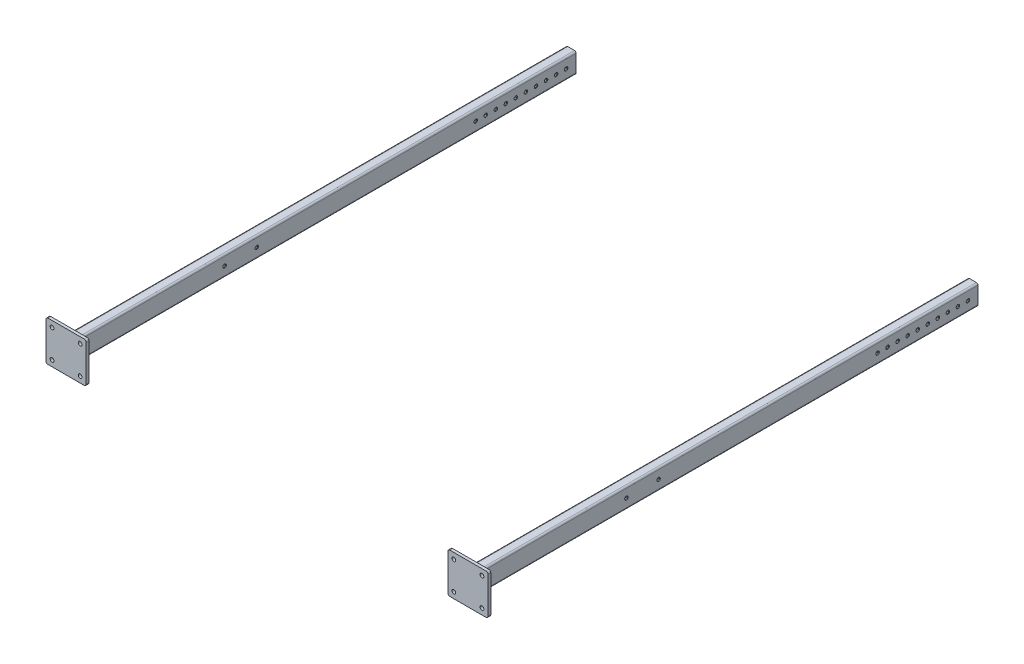
SolidWorks part; units mm, degrees
ref_plane "Front Plane" through (0, 0, 0) normal (0, 0, 1) x (1, 0, 0)
ref_plane "Top Plane" through (0, 0, 0) normal (0, 1, 0) x (1, 0, 0)
ref_plane "Right Plane" through (0, 0, 0) normal (1, 0, 0) x (0, 0, -1)
other "Configuration Table"
sketch3d "3DSketch1"
  line L0 (-1000, 0, 0) -> (1000, 0, 0) construction
  line L1 (-1000, 0, 0) -> (-1000, 0, -2500)
  line L2 (1000, 0, 0) -> (1000, 0, -2500)
  point P4 (0, 0, 0)
  dimension "D1" = 2000
  dimension "D2" = 2500
other "Gb／6728-1986 rectangular hollow section 100 X 50 X 4 (1)"
ref_plane "Plane1" through (-1000, 0, 0) normal (0, 0, -1) x (1, 0, 0)
sketch "Sketch12" plane through (-1000, 0, 0) normal (0, 0, -1) x (1, 0, 0)
  line L0 (-17, -46) -> (17, -46)
  line L1 (-21, -42) -> (-21, 42)
  line L2 (17, 46) -> (-17, 46)
  line L3 (21, 42) -> (21, -42)
  line L4 (-17, -50) -> (17, -50)
  line L5 (-25, -42) -> (-25, 42)
  line L6 (17, 50) -> (-17, 50)
  line L7 (25, 42) -> (25, -42)
  arc A0 (25, 42) -> (17, 50) centre (17, 42) ccw
  arc A1 (17, -50) -> (25, -42) centre (17, -42) ccw
  arc A2 (-25, -42) -> (-17, -50) centre (-17, -42) ccw
  arc A3 (-17, 50) -> (-25, 42) centre (-17, 42) ccw
  arc A4 (-17, 46) -> (-21, 42) centre (-17, 42) ccw
  arc A5 (21, 42) -> (17, 46) centre (17, 42) ccw
  arc A6 (17, -46) -> (21, -42) centre (17, -42) ccw
  arc A7 (-21, -42) -> (-17, -46) centre (-17, -42) ccw
  point P0 (0, 50)
  point P1 (25, 0)
  point P2 (0, -50)
  point P3 (-25, 0)
  point P4 (-25, 50)
  point P5 (25, 50)
  point P6 (25, -50)
  point P7 (-25, -50)
  point P8 (0, 0)
  point P33 (0, 0)
  dimension "D1" = 8
  dimension "Thickness" = 4
  dimension "V_leg" = 100
  dimension "H_leg" = 50
sketch "Sketch5" plane through (0, 0, 0) normal (0, 0, 1) x (1, 0, 0)
  line L1 (-1100, -100) -> (-900, -100)
  line L2 (-1100, -100) -> (-1100, 100)
  line L3 (-1100, 100) -> (-900, 100)
  line L4 (-900, -100) -> (-900, 100)
  line L5 (-1100, -100) -> (-900, 100) construction
  line L6 (-1100, 100) -> (-900, -100) construction
  point P0 (-1000, 0)
  dimension "D1" = 200
  dimension "D2" = 200
extrude "Boss-Extrude1" add sketch "Sketch5" along normal blind 14 separate body
ref_plane "Plane2" through (0, 0, 0) normal (-1, 0, 0) x (0, 0, 1)
fillet "Fillet1" radius 10 4 edges at (-1100, -100, 7) (-900, -100, 7) (-900, 100, 7) (-1100, 100, 7)
hole_wizard "M16 Clearance Hole1" positions "Sketch7" profile "Sketch9" hole size "M16" standard "GB" end condition through all
sketch "Sketch7" plane through (0, 0, 0) normal (0, 0, -1) x (-1, 0, 0)
  line L0 (1000, 100) -> (1000, -100) construction
  line L1 (910, 100) -> (1090, 100) construction
  line L2 (1090, -100) -> (910, -100) construction
  line L4 (900, 0) -> (1100, 0) construction
  line L5 (900, -90) -> (900, 90) construction
  line L6 (1100, 90) -> (1100, -90) construction
  point P0 (1070, 70)
  point P2 (1070, -70)
  point P4 (930, -70)
  point P6 (930, 70)
  dimension "D1" = 140
  dimension "D2" = 140
sketch "Sketch9" plane through (-1070, 70, 0) normal (1, 0, 0) x (0, 1, 0)
  line L0 (0, 0) -> (0, 14)
  line L1 (0, 14) -> (9.5, 14)
  line L2 (9.5, 14) -> (9.5, 0)
  line L5 (9.5, 0) -> (0, 0)
  line L11 (0, -6.35) -> (0, 107.95) construction
  dimension "通孔孔直径" = 19
  dimension "通孔孔深度" = 14
mirror "Mirror1" about plane through (0, 0, 0) normal (-1, 0, 0) of bodies 110 108
sketch "Sketch10" plane through (975, 0, 0) normal (-1, 0, 0) x (0, 0, 1)
  line L0 (-2500, 0) -> (0, 0) construction
  line L1 (0, 90) -> (0, -90) construction
  line L2 (-950, -100) -> (-750, -100)
  line L3 (-950, -100) -> (-950, 100)
  line L4 (-950, 100) -> (-750, 100)
  line L5 (-750, -100) -> (-750, 100)
  line L6 (-950, -100) -> (-750, 100) construction
  line L7 (-950, 100) -> (-750, -100) construction
  point P4 (-850, 0)
  dimension "D1" = 200
  dimension "D2" = 200
  dimension "D3" = 750
extrude "Boss-Extrude2" [suppressed] add sketch "Sketch10" along normal blind 14 separate body
fillet "Fillet2" [suppressed] radius 10
hole_wizard "M16 Tapped Hole2" positions "Sketch11" profile "草图12" tap size "M16" standard "GB"
sketch "Sketch11" [suppressed] plane through (961, 0, 0) normal (-1, 0, 0) x (0, 0, 1)
  line L0 (-850, 100) -> (-850, -100) construction
  line L1 (-760, 100) -> (-940, 100) construction
  line L2 (-940, -100) -> (-760, -100) construction
  line L4 (-850, 0) -> (-811.3519, 0) construction
  line L5 (0, 0) -> (-2500, 0) construction
  point P0 (-920, 70)
  point P2 (-780, 70)
  point P4 (-780, -63.6766)
  point P6 (-920, -70)
  dimension "D1" = 140
  dimension "D2" = 140
sketch "草图12" plane through (961, 70, -920) normal (0, 1, 0) x (0, 0, 1)
  line L0 (0, 0) -> (0, 139)
  line L1 (0, 139) -> (7, 139)
  line L2 (7, 139) -> (7, 0)
  line L5 (7, 0) -> (0, 0)
  line L11 (0, -6.35) -> (0, 107.95) construction
  dimension "通孔螺纹孔钻头直径" = 14
  dimension "通孔螺纹孔钻头深度" = 139
mirror "Mirror2" [suppressed] about plane through (0, 0, 0) normal (-1, 0, 0)
hole_wizard "M16 Clearance Hole3" positions "Sketch13" profile "Sketch14" hole size "M16" standard "GB" end condition through all
sketch "Sketch13" plane through (1025, 0, 0) normal (1, 0, 0) x (0, 0, -1)
  line L0 (0, 0) -> (2500, 0) construction
  line L1 (2500, 42) -> (2500, -42) construction
  point P0 (2450, 0)
  dimension "D1" = 50
sketch "Sketch14" plane through (1025, 0, -2450) normal (0, 1, 0) x (0, 0, -1)
  line L0 (0, 0) -> (0, 2125)
  line L1 (0, 2125) -> (8.75, 2125)
  line L2 (8.75, 2125) -> (8.75, 0)
  line L5 (8.75, 0) -> (0, 0)
  line L11 (0, -6.35) -> (0, 107.95) construction
  dimension "通孔孔直径" = 17.5
  dimension "通孔孔深度" = 2125
pattern_linear "LPattern1" count 10 spacing 50 along (0, 0, 1) of "M16 Clearance Hole3"
hole_wizard "M16 Clearance Hole4" positions "Sketch15" profile "Sketch16" hole size "M16" standard "GB" end condition through all
sketch "Sketch15" plane through (-1025, 0, 0) normal (-1, 0, 0) x (0, 0, 1)
  line L0 (0, 0) -> (-600, 0) construction
  line L2 (0, -42) -> (0, 42) construction
  point P0 (-750, 0)
  point P2 (-910, 0)
  dimension "D1" = 600
  dimension "D2" = 160
  dimension "D3" = 750
sketch "Sketch16" plane through (-1025, 0, -750) normal (0, 1, 0) x (0, 0, 1)
  line L0 (0, 0) -> (0, 2125)
  line L1 (0, 2125) -> (8.75, 2125)
  line L2 (8.75, 2125) -> (8.75, 0)
  line L5 (8.75, 0) -> (0, 0)
  line L11 (0, -6.35) -> (0, 107.95) construction
  dimension "通孔孔直径" = 17.5
  dimension "通孔孔深度" = 2125
